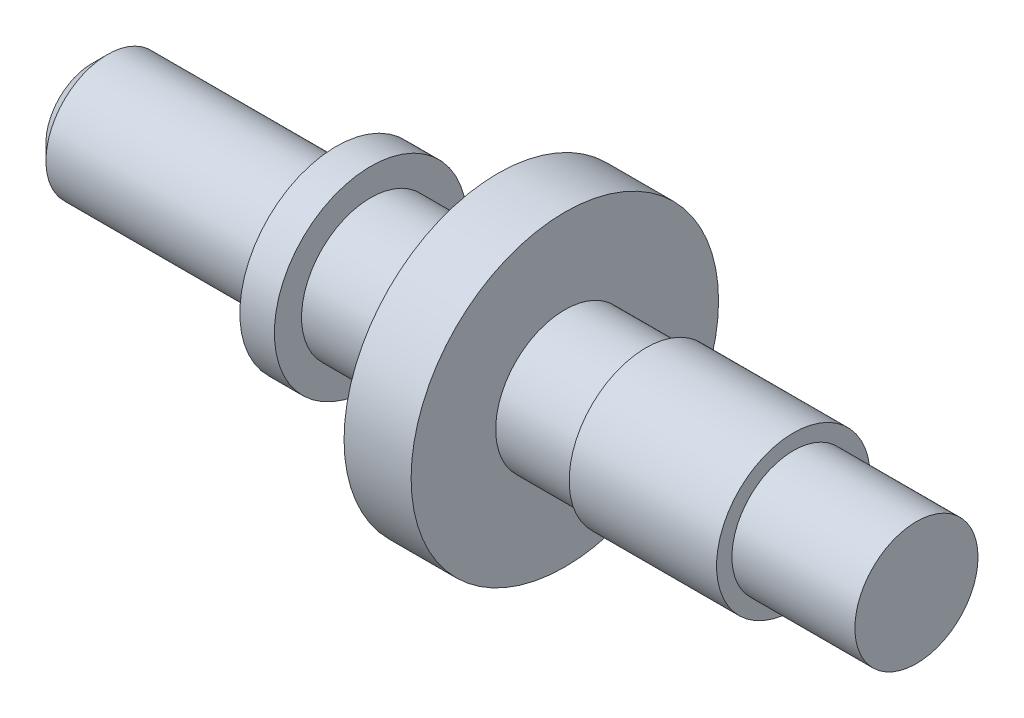
from build123d import *


with BuildPart() as part:
    # Model → Revolve1 (revolve)
    with BuildSketch(Plane.XY, mode=Mode.PRIVATE) as revolve1_sk:
        Polygon((49.51331086, -13.474001866), (49.517097509, -14.469395389), (57.517097509, -14.469395389), (57.517097509, -18.474001866), (3.884490088, -18.474001866), (3.884490088, -15.474001866), (4.884490088, -14.474001866), (11.769027201, -14.474001866), (19.769026262, -14.474001866), (19.769027201, -12.204912355), (22.015056766, -12.204912355), (22.015056766, -13.974001866), (30.280660424, -13.974001866), (30.280660424, -8.474001866), (34.643062355, -8.474001866), (34.643062355, -13.974001866), (39.923864692, -13.974001866), (39.923864692, -13.474001866), align=None)
    revolve(revolve1_sk.sketch.rotate(Axis((3.884490088, -18.474001866, 0), (-1, 0, 0)), 90), axis=Axis((3.884490088, -18.474001866, 0), (-1, 0, 0)))


solid = part.part
